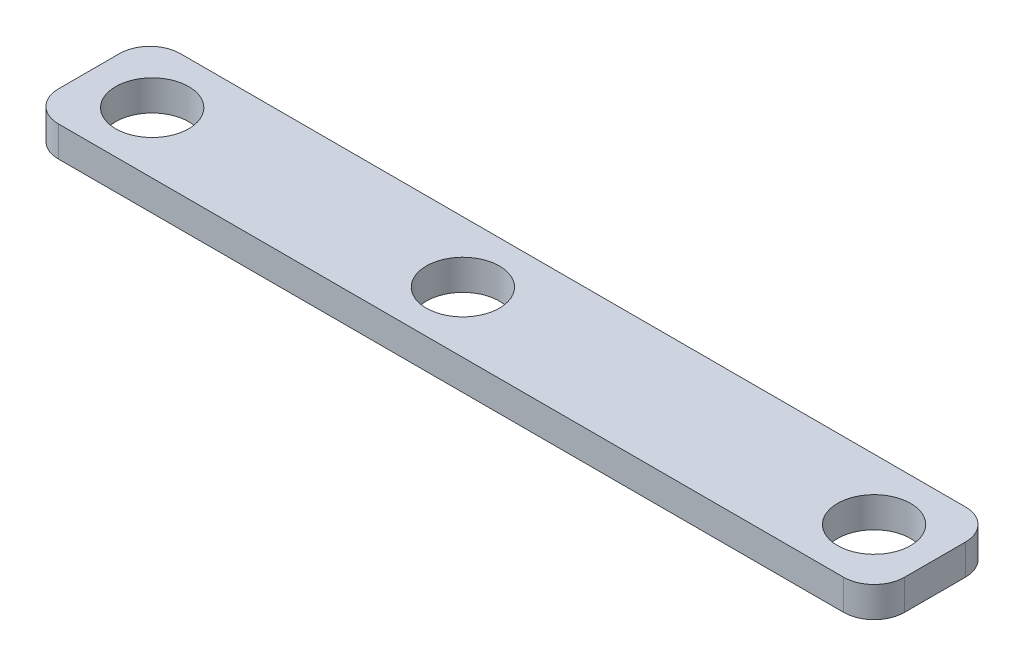
from build123d import *

# Parameters (mm, degrees)
SKETCH1_W           = 300
SKETCH1_H           = 40
SKETCH1_R           = 12
BOSS_EXTRUDE1_DEPTH = 10
SKETCH2_W           = 22.25652502
SKETCH2_H           = 40
CUT_EXTRUDE1_DEPTH  = 10
FILLET1_R           = 10


with BuildPart() as part:
    # Sketch1 → Boss-Extrude1 (new body)
    with BuildSketch(Plane(origin=(0, 0, 0), x_dir=(1, 0, 0), z_dir=(0, 1, 0))):
        Rectangle(SKETCH1_W, SKETCH1_H)
        with Locations(Location((130, 0, 0), (0, 0, 270))):
            Circle(SKETCH1_R, mode=Mode.SUBTRACT)
        with Locations(Location((-5, 0, 0), (0, 0, 270))):
            Circle(SKETCH1_R, mode=Mode.SUBTRACT)
        with Locations(Location((-107, 0, 0), (0, 0, 270))):
            Circle(SKETCH1_R, mode=Mode.SUBTRACT)
    extrude(amount=BOSS_EXTRUDE1_DEPTH)

    # Sketch2 → Cut-Extrude1 (cut)
    with BuildSketch(Plane(origin=(0, 10, 0), x_dir=(1, 0, 0), z_dir=(0, 1, 0))):
        with Locations((-138.87173749, 0)):
            Rectangle(SKETCH2_W, SKETCH2_H)
    extrude(amount=-CUT_EXTRUDE1_DEPTH, mode=Mode.SUBTRACT)

    # Fillet1
    fillet1_edges = [part.edges().sort_by_distance(p)[0] for p in [
        (-127.74347498, 5, -20),
        (-127.74347498, 5, 20),
        (150, 5, 20),
        (150, 5, -20),
    ]]
    fillet(fillet1_edges, radius=FILLET1_R)


solid = part.part
